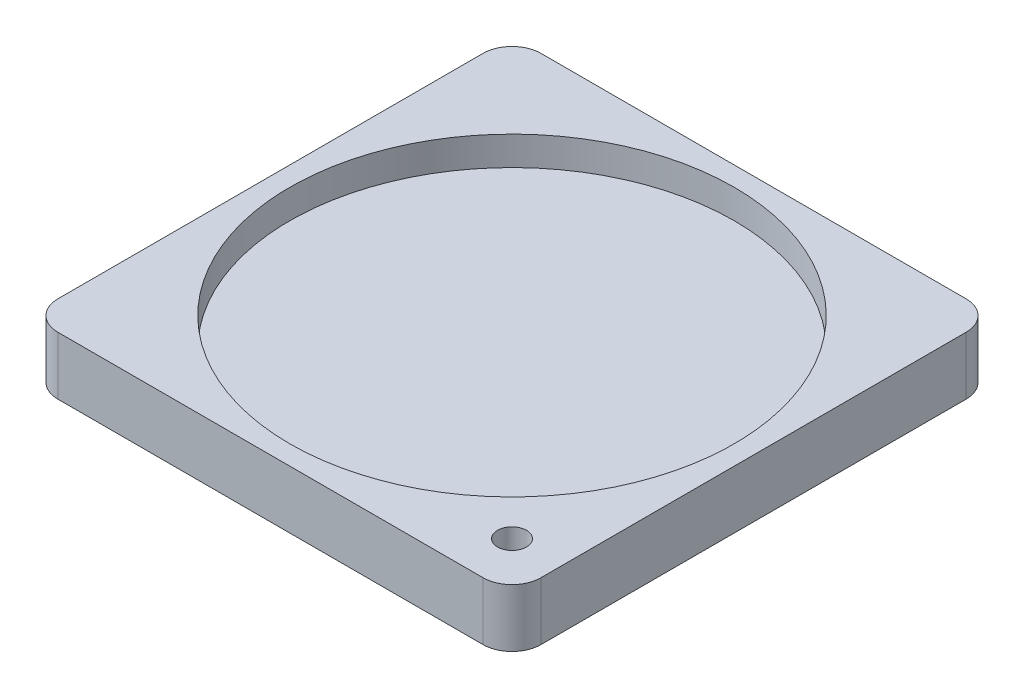
SolidWorks part; units mm, degrees
ref_plane "Front Plane" through (0, 0, 0) normal (0, 0, 1) x (1, 0, 0)
ref_plane "Top Plane" through (0, 0, 0) normal (0, 1, 0) x (1, 0, 0)
ref_plane "Right Plane" through (0, 0, 0) normal (1, 0, 0) x (0, 0, -1)
sketch "Sketch1" plane through (0, 0, 0) normal (0, 1, 0) x (1, 0, 0)
  line L1 (-25, -25) -> (25, -25)
  line L2 (-25, -25) -> (-25, 25)
  line L3 (-25, 25) -> (25, 25)
  line L4 (25, -25) -> (25, 25)
  line L5 (-25, -25) -> (25, 25) construction
  line L6 (-25, 25) -> (25, -25) construction
  point P0 (0, 0)
  dimension "D1" = 50
  dimension "D2" = 50
extrude "Boss-Extrude1" add sketch "Sketch1" along normal blind 10
sketch "Sketch2" plane through (0, 10, 0) normal (0, 1, 0) x (1, 0, 0)
  circle A0 centre (0, 0) radius 23
  dimension "D1" = 46
extrude "Cut-Extrude1" cut sketch "Sketch2" against normal blind 3
sketch "Sketch3" plane through (0, 10, 0) normal (0, 1, 0) x (1, 0, 0)
  line L2 (25, -25) -> (25, 25) construction
  line L3 (-25, -25) -> (25, -25) construction
  circle A1 centre (20, -20) radius 1.5
  dimension "D1" = 3
  dimension "D2" = 5
  dimension "D3" = 5
extrude "Cut-Extrude2" cut sketch "Sketch3" against normal blind 3
sketch "Sketch4" plane through (0, 0, 25) normal (0, 0, 1) x (1, 0, 0)
  line L0 (-25, 10) -> (-25, 0) construction
  line L1 (-25, 0) -> (25, 0)
  line L2 (-25, 0) -> (-25, 4)
  line L3 (-25, 4) -> (25, 4)
  line L4 (25, 0) -> (25, 4)
  line L5 (-25, 0) -> (25, 0) construction
  line L6 (25, 10) -> (25, 0) construction
  dimension "D1" = 4
extrude "Cut-Extrude3" cut sketch "Sketch4" against normal blind 76
fillet "Fillet1" radius 3 4 edges at (-25, 7, -25) (25, 7, -25) (25, 7, 25) (-25, 7, 25)
sketch "Sketch5" plane through (0, 4, 0) normal (0, -1, 0) x (1, 0, 0)
  line L1 (-16, -16) -> (16, -16) construction
  line L2 (-16, -16) -> (-16, 16) construction
  line L3 (-16, 16) -> (16, 16) construction
  line L4 (16, -16) -> (16, 16) construction
  line L5 (-16, -16) -> (16, 16) construction
  line L6 (-16, 16) -> (16, -16) construction
  circle A0 centre (-16, 16) radius 1.5
  circle A1 centre (16, 16) radius 1.5
  circle A3 centre (-16, -16) radius 1.5
  circle A4 centre (16, -16) radius 1.5
  point P0 (0, 0)
  dimension "D3" = 3
  dimension "D4" = 3
  dimension "D5" = 3
  dimension "D6" = 3
  dimension "D1" = 32
  dimension "D2" = 32
extrude "Cut-Extrude4" cut sketch "Sketch5" against normal blind 1
